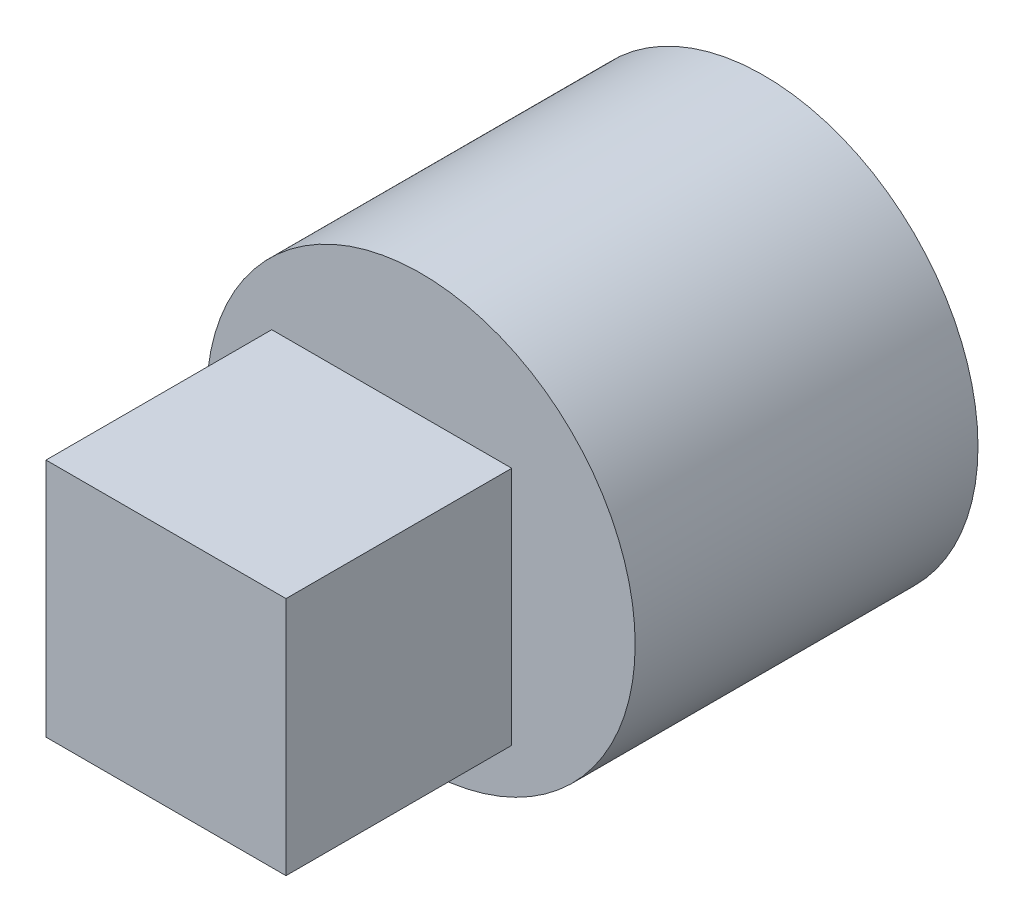
from build123d import *

# Parameters (mm, degrees)
SKETCH_1_R          = 12.5
EXTRUDE_1_DEPTH     = 20
SKETCH_2_W          = 8.5
SKETCH_2_H          = 8.5
EXTRUDE_2_DEPTH     = 1.7
SKETCH_3_W          = 14
SKETCH_3_H          = 14
EXTRUDE_3_DEPTH     = 13.17
SKETCH_4_R          = 10
CUT_EXTRUDE_1_DEPTH = 15
CHAMFER_1_SIZE      = 0.5


with BuildPart() as part:
    # 草图1 → 凸台-拉伸1 (new body)
    with BuildSketch(Plane.XY):
        Circle(SKETCH_1_R)
    extrude(amount=EXTRUDE_1_DEPTH)

    # 草图2 → 凸台-拉伸2 (add)
    with BuildSketch(Plane.XY.offset(20)):
        Rectangle(SKETCH_2_W, SKETCH_2_H)
    extrude(amount=EXTRUDE_2_DEPTH)

    # 草图3 → 凸台-拉伸3 (add)
    with BuildSketch(Plane.XY.offset(21.7)):
        Rectangle(SKETCH_3_W, SKETCH_3_H)
    extrude(amount=EXTRUDE_3_DEPTH)

    # 草图4 → 切除-拉伸1 (cut)
    with BuildSketch(Plane(origin=(0, 0, 0), x_dir=(-1, 0, 0), z_dir=(0, 0, -1))):
        Circle(SKETCH_4_R)
    extrude(amount=-CUT_EXTRUDE_1_DEPTH, mode=Mode.SUBTRACT)

    # 倒角1
    chamfer_1_edges = [part.edges().sort_by_distance(p)[0] for p in [
        (4.25, 0, 20),
        (0, 4.25, 20),
        (-4.25, 0, 20),
        (0, -4.25, 20),
    ]]
    chamfer(chamfer_1_edges, length=CHAMFER_1_SIZE)


solid = part.part
